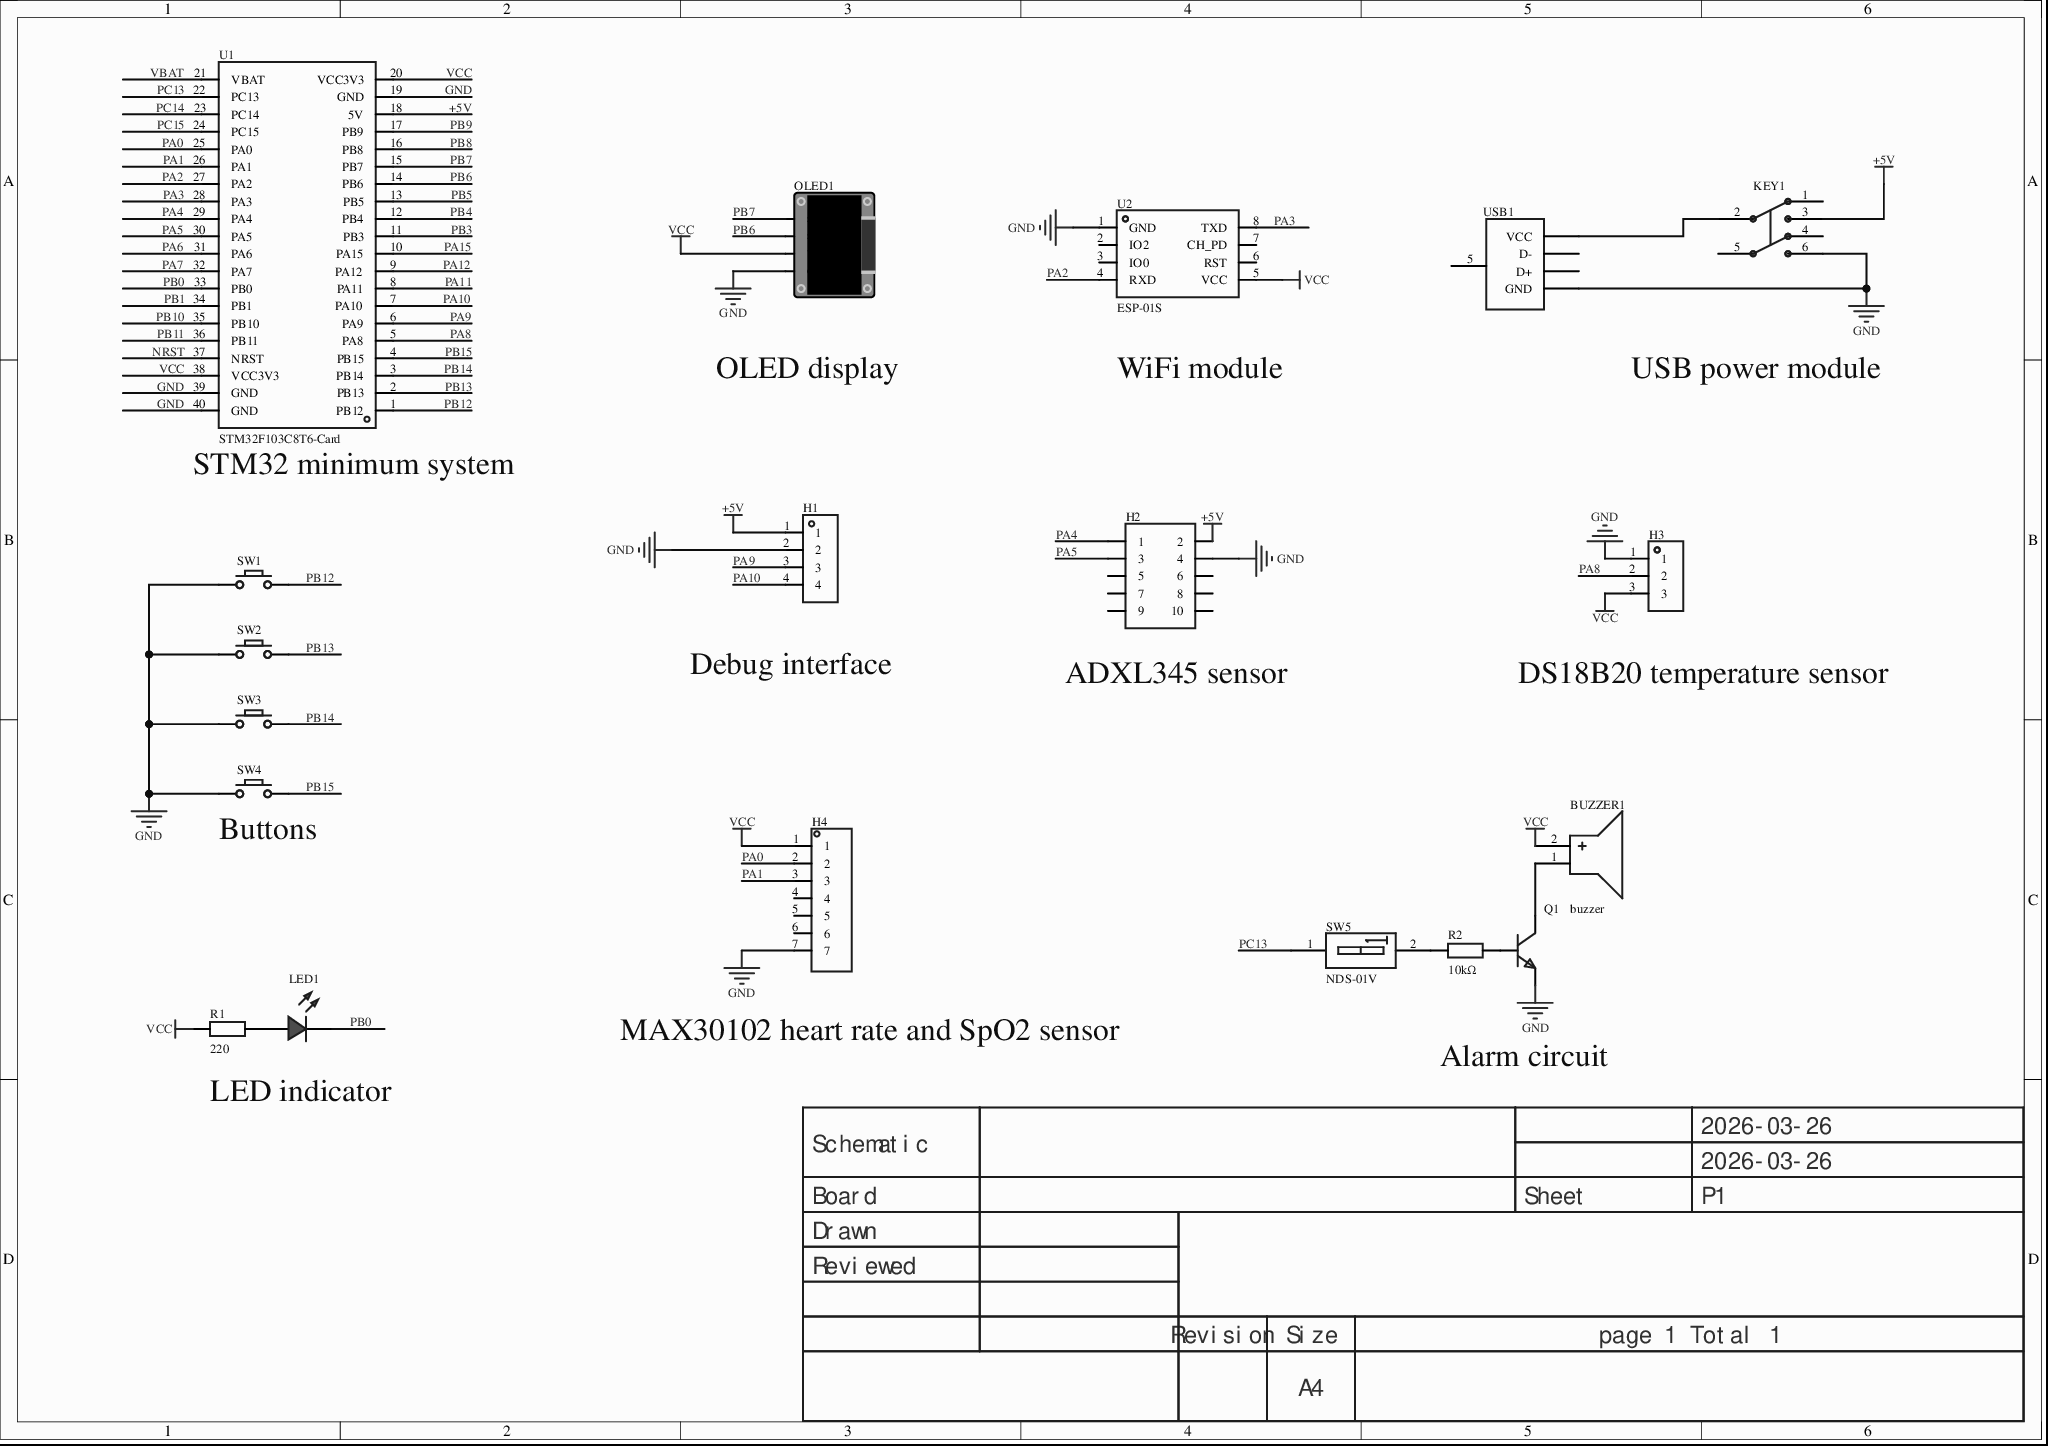
[diagram p0: MISC51590-3.schdoc]
# Altium project MISC51590-2.PrjPcb
1 sheet, 19 parts. Net scope: global (net labels, ports and power ports of the same name join across sheets).
Board file: MISC51590.pcbdoc

## Sheet MISC51590-3.schdoc
size 297 x 209 mm; Version: V1.0; @Project Name: MISC51590; @Page Count: 1; @Update Date: 2026-03-26; @Create Date: 2026-03-26; @Schematic Name: MISC51590; @Page No: 1; @Create Time: 18:58:15; @Update Time: 22:44:58; @Board Name: MISC51590

### Parts
BUZZER1  buzzer  [BUZ-TH_BD12.0-P6.00-D0.9-RD]
H1  (no value)  [HDR-TH_4P-P2.54-V-M]
H2  (no value)  [HDR-TH_10P-P2.54-V-F-R2-C5-S2.54]
H3  (no value)  [HDR-TH_3P-P2.54-V-F]
H4  (no value)  [HDR-TH_7P-P2.54-V-F]
KEY1  Non-self-locking switch 8.5×8.5 silent  [SW-TH_6P-L8.5-W8.5-P2.54]  (value not drawn)
LED1  (no value)  [LED_TH-3mm]
OLED1  (no value)  [0.96OLED_4P]
Q1  (no value)  [S8050_TO_92]
R1  220  [Res_1/8W]
R2  10kΩ  [Res_1/8W]
SW1  (no value)  [Key_TH_3.5x6x4.3]
SW2  (no value)  [Key_TH_3.5x6x4.3]
SW3  (no value)  [Key_TH_3.5x6x4.3]
SW4  (no value)  [Key_TH_3.5x6x4.3]
SW5  NDS-01V  [SW-TH_2P-L3.9-W9.9-P2.54-LS7.6]
U1  STM32F103C8T6-Card  [CONN-TH_L53.3-W22.9_STM32F103C8T6-CARD]
U2  ESP-01S  [WIFIM-TH_ESP-01S]
USB1  (no value)  [USB_ Type-B]

### Nets
+5V: H1.1 H2.2 KEY1.3 U1.18(5V)
GND: H1.2 H2.4 H3.1 H4.7 KEY1.6 OLED1.1(GND) Q1.1(E) SW1.A SW2.A SW3.A SW4.A U1.19(GND) U1.39(GND) U1.40(GND) U2.1(GND) USB1.4(GND)
VCC: BUZZER1.2(+) H3.3 H4.1 OLED1.2(VCC) R1.1 U1.20(VCC3V3) U1.38(VCC3V3) U2.5(VCC)
NRST: U1.37(NRST)
PA0: H4.2 U1.25(PA0)
PA1: H4.3 U1.26(PA1)
PA2: U1.27(PA2) U2.4(RXD)
PA3: U1.28(PA3) U2.8(TXD)
PA4: H2.1 U1.29(PA4)
PA5: H2.3 U1.30(PA5)
PA6: U1.31(PA6)
PA7: U1.32(PA7)
PA8: H3.2 U1.5(PA8)
PA9: H1.3 U1.6(PA9)
PA10: H1.4 U1.7(PA10)
PA11: U1.8(PA11)
PA12: U1.9(PA12)
PA15: U1.10(PA15)
PB0: LED1.2(A) U1.33(PB0)
PB1: U1.34(PB1)
PB3: U1.11(PB3)
PB4: U1.12(PB4)
PB5: U1.13(PB5)
PB6: OLED1.3(SCL) U1.14(PB6)
PB7: OLED1.4(SDA) U1.15(PB7)
PB8: U1.16(PB8)
PB9: U1.17(PB9)
PB10: U1.35(PB10)
PB11: U1.36(PB11)
PB12: SW1.B U1.1(PB12)
PB13: SW2.B U1.2(PB13)
PB14: SW3.B U1.3(PB14)
PB15: SW4.B U1.4(PB15)
PC13: SW5.1(A1) U1.22(PC13)
PC14: U1.23(PC14)
PC15: U1.24(PC15)
VBAT: U1.21(VBAT)
NetBUZZER1_1: BUZZER1.1(-) Q1.3(C)
NetKEY1_2: KEY1.2 USB1.1(VCC)
NetLED1_1: LED1.1(C) R1.2
NetQ1_2: Q1.2(B) R2.2
NetR2_1: R2.1 SW5.2(A2)

Not connected (* = marked no-connect by the designer): H2 5 6 7 8 9 10; H4 4 5 6; KEY1 1 4 5; U2 2(IO2)* 3(IO0)* 6(RST)* 7(CH_PD)*; USB1 2(D-)* 3(D+)* 5(SH1)

### Notes on the sheet
- OLED display
- WiFi module
- USB power module
- (near U1) STM32 minimum system
- (near H1) Debug interface
- (near H2) ADXL345 sensor
- (near H3) DS18B20 temperature sensor
- (near SW4) Buttons
- (near H4) MAX30102 heart rate and SpO2 sensor
- LED indicator
- Alarm circuit
- 2026-03-26
- Schematic
- Board
- Sheet
- P1
- Drawn
- Reviewed
- Revision
- Size
- A4
- page 1 Total 1

### Library data of the parts
BUZZER1 = buzzer: AddInBom: yes; ModelId: af17e4151ed84fc2a628230bf23763630819f05c4eef4c71ace90d822a990e87; ModelTransform: 472.44,472.176,0,270,0,0,0,0,-196.85; Symbol: BUZZER; Device: buzzer; LCSC Part Name: buzzer; SupplierPart: C9900014030; ManufacturerPart: buzzer; Supplier Footprint: buzzer; JLCPCB Part Class: Extended Part; Supplier: LCSC; ConvertToPcb: yes; FootprintName: BUZ-TH_BD12.0-P6.00-D0.9-RD; ModelName: BUZ-TH_BD12.0-P6.00-D0.9-RD
H1 = HDR-M_2.54_1x4P: Symbol: PZ254V-11-04P; ConvertToPcb: yes; ModelId: 112f4d05e8d64e99ab9a333894bea4f90819f05c4eef4c71ace90d822a990e87; ModelName: HDR-TH_4P-P2.54-M-LI-1X4P; ModelTransform: 399.999,104.7242,0,0,0,0,0,0,-118.11; Device: HDR-M_2.54_1x4P; AddInBom: yes; SupplierPart: C492403; Supplier Footprint: 插件; FootprintName: HDR-TH_4P-P2.54-V-M
H2 = HDR-F_2.54_2x5: Symbol: HDR-F-2.54_2x5; ConvertToPcb: yes; ModelId: 86e5d65f54dd476391caab3fdb9168240819f05c4eef4c71ace90d822a990e87; ModelName: HDR2.54-F-LI-2X5P; ModelTransform: 499.999,200,0,0,0,0,0,0,-118.11; Device: HDR-F_2.54_2x5; AddInBom: yes; SupplierPart: C92270; Supplier Footprint: 插件; FootprintName: HDR-TH_10P-P2.54-V-F-R2-C5-S2.54
H3 = HDR-F_2.54_1x3P: Symbol: PM254V-11-03-H85; ConvertToPcb: yes; ModelId: f3b3cc5aae9641bf9e56fc160cef875b; ModelName: HDR2.54-F-LI-1X3P; ModelTransform: 299.9994,100,0,0,0,0,0,0,-118.11; Device: HDR-F_2.54_1x3P; AddInBom: yes; SupplierPart: C541850; Supplier Footprint: 插件; FootprintName: HDR-TH_3P-P2.54-V-F
H4 = HDR-F_2.54_1x7P: Symbol: 220S-1*7P H=8.5MM Ytype Gold-plated; ConvertToPcb: yes; ModelId: 4c31987253bc43b9b52c17be2a6d3f910819f05c4eef4c71ace90d822a990e87; ModelName: HDR-TH_7P-P2.54-F-LI-1X7P; ModelTransform: 715.7466,94.488,0,0,0,0,0,0,-118.11; Device: HDR-F_2.54_1x7P; AddInBom: yes; SupplierPart: C124418; Supplier Footprint: 插件; FootprintName: HDR-TH_7P-P2.54-V-F
KEY1 = 无自锁开关 8.5×8.5 无声: 6脚，8.5×8.5; Symbol: No self-locking switch 8.5×8.5 silent; AddInBom: yes; ModelId: 4c72b3966b92446eb355e1bd0fb4f8800819f05c4eef4c71ace90d822a990e87; ModelTransform: 342.519,334.645,0,180,0,0,0,0,-137.795; Device: Non-self-locking switch 8.5×8.5 silent; LCSC Part Name: 无自锁开关 8.5×8.5  无声; SupplierPart: C26228; ManufacturerPart: 无自锁开关 8.5×8.5 无声; Supplier Footprint: 插件; JLCPCB Part Class: Extended Part; Supplier: LCSC; ConvertToPcb: yes; FootprintName: SW-TH_6P-L8.5-W8.5-P2.54; ModelName: SW-TH_6P-L8.5-W8.5-P2.54
LED1 = LED_TH-R_3mm: ConvertToPcb: yes; ModelId: a497c992633541038a38947cdc58012f0819f05c4eef4c71ace90d822a990e87; ModelName: LED-TH-3mm_R; ModelTransform: 141.274,153.327,0,0,0,0,-5.984,0,-137.795; Symbol: LED_TH-R; Device: LED_TH-R_3mm; AddInBom: yes; FootprintName: LED_TH-3mm; Supplier Footprint: 插件
OLED1 = 0.96OLED模块_4P: Symbol: 0.96OLED module_4P; ConvertToPcb: yes; ModelId: 79c000fdb68d45a296c2e9bedf4f9055; ModelTransform: 1393.69792,1318.895,0,0,0,0,0,-560.079,-137.795; Device: 0.96OLED module_4P; AddInBom: yes; FootprintName: 0.96OLED_4P; Supplier Footprint: 插件; ModelName: 0.96OLED_4P
Q1 = S8050_TO_NPN: ConvertToPcb: yes; ModelId: aafe8e06f2154e7c93506efd0d6632dd; ModelName: TO-92-3_L4.9-W3.7-P1.27-L; ModelTransform: 180.78,141.44,417.3,0,0,0,0,0,-200; Symbol: S8050_TO_NPN; Device: S8050_TO_NPN; AddInBom: yes; Supplier Footprint: TO-92; FootprintName: S8050_TO_92
R1 R2 = Res_AXIAL-1/8W: Symbol: Resistor; ConvertToPcb: yes; ModelId: b2b5ae7ae4c642178fe0039925c86a3f; ModelName: RES-TH_BD1.8-L3.2-P7.20-D0.4; ModelTransform: 282.86,66.88,253.09,0,0,0,0,0,-191; Device: Res_AXIAL-1/8W; AddInBom: yes; Supplier Footprint: 轴向引线; FootprintName: Res_1/8W
  R1: Value: 220
  R2: Value: 10kΩ
SW1-SW4 = Key_TH_3.5x6x4.3: ConvertToPcb: yes; ModelId: c3523f9014d949d7ba5445190a3178990819f05c4eef4c71ace90d822a990e87; ModelName: SW-TH_L6.0-W3.5-H5.0-P6.5; ModelTransform: 308.49,137.8,335.08,0,0,0,0,0,-129.92; Symbol: Key_TH_3.5x6x4.3; Device: Key_TH_3.5x6x4.3; AddInBom: yes; Supplier Footprint: 插件; FootprintName: Key_TH_3.5x6x4.3
SW5 = NDS-01V_C501305: NDS-01V_C501305 co high-lever forward toggle; AddInBom: yes; ModelId: a6fe51954c31461ebc9e88beb6e51f3d0819f05c4eef4c71ace90d822a990e87; ModelName: SW-TH_L4.0-W9.9-H5.4-P2.54-B; ModelTransform: 161.417,389.763,0,270,0,0,0,0,-125.984; Symbol: NDS-01V; Device: NDS-01V_C501305; LCSC Part Name: 拨码开关; SupplierPart: C501305; ManufacturerPart: NDS-01V; Supplier Footprint: DIP; JLCPCB Part Class: Extended Part; Supplier: LCSC; ConvertToPcb: yes; FootprintName: SW-TH_2P-L3.9-W9.9-P2.54-LS7.6
U1 = STM32F103C8T6-Card: AddInBom: yes; Symbol: STM32F103C8T6-CARD; Device: STM32F103C8T6-Card; LCSC Part Name: STM32F103C8T6-Card; SupplierPart: C9900077949; ManufacturerPart: STM32F103C8T6-Card; Supplier Footprint: 插件; Supplier: LCSC; ConvertToPcb: yes; FootprintName: CONN-TH_L53.3-W22.9_STM32F103C8T6-CARD
U2 = ESP-01S_C111009: AddInBom: yes; ModelId: eb7175da78ae48b3b1568cfe3027405f0819f05c4eef4c71ace90d822a990e87; ModelTransform: 582.676,976.37608,0,0,0,0,0,388.346,-118.11; Symbol: ESP-01S; Device: ESP-01S_C111009; LCSC Part Name: ESP-01S; SupplierPart: C111009; ManufacturerPart: ESP-01S; Supplier Footprint: -; JLCPCB Part Class: Extended Part; Supplier: LCSC; ConvertToPcb: yes; FootprintName: WIFIM-TH_ESP-01S; ModelName: WIFIM-TH_ESP-01S
USB1 = USB_ Type-B: ConvertToPcb: yes; ModelId: bbf32347d5be4dcea8001c0804ac390e0819f05c4eef4c71ace90d822a990e87; ModelName: USB-B_TH_BF90; ModelTransform: 547.99,637.8,543.15,0,0,0,0,0,-125.98; Symbol: USB_ Type-B; Device: USB_ Type-B; AddInBom: yes; Supplier Footprint: 插件; FootprintName: USB_ Type-B